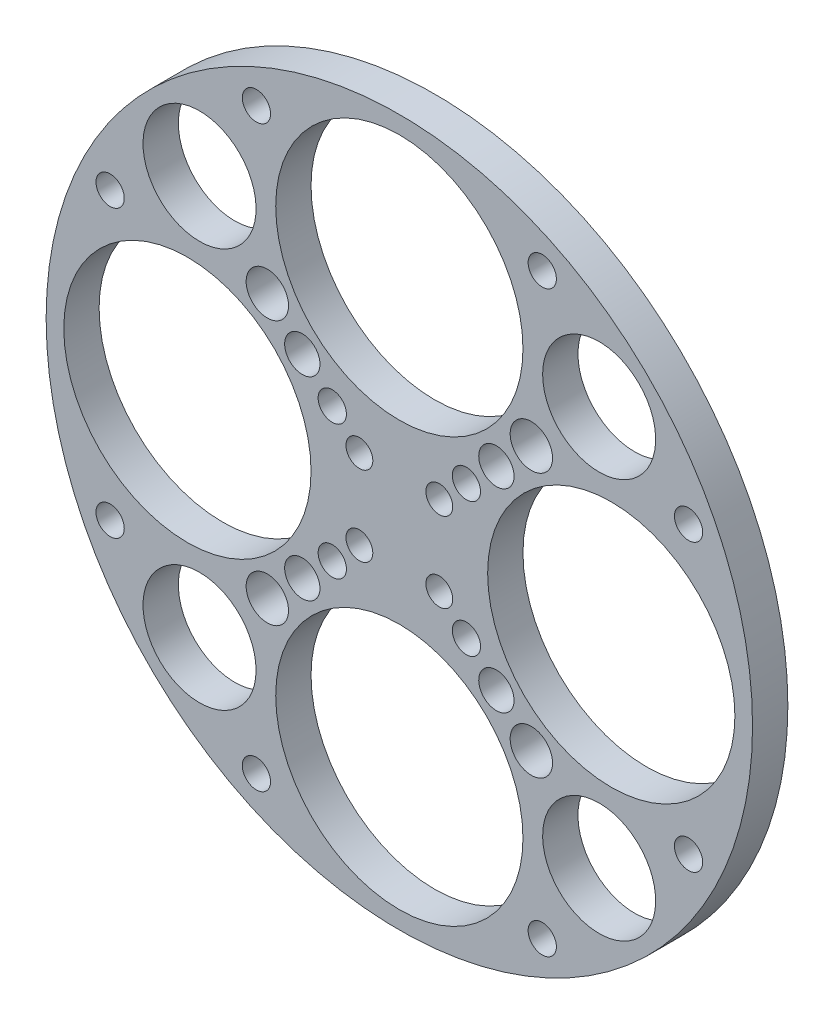
SolidWorks part; units mm, degrees
material "Acrylic (Medium-high impact)"
ref_plane "Front Plane" through (0, 0, 0) normal (0, 0, 1) x (1, 0, 0)
ref_plane "Top Plane" through (0, 0, 0) normal (0, 1, 0) x (1, 0, 0)
ref_plane "Right Plane" through (0, 0, 0) normal (1, 0, 0) x (0, 0, -1)
sketch "Sketch1" plane through (0, 0, 0) normal (0, 0, 1) x (1, 0, 0)
  circle A0 centre (0, 0) radius 50
  dimension "D1" = 100
extrude "Boss-Extrude1" add sketch "Sketch1" along normal blind 5
sketch "Sketch2" plane through (0, 0, 0) normal (0, 0, -1) x (-1, 0, 0)
  line L0 (0, 0) -> (0, 50) construction
  line L1 (-5.6569, 5.6569) -> (0, 0) construction
  circle A0 centre (-5.6569, 5.6569) radius 1.9
  circle A1 centre (0, 0) radius 50 construction
  dimension "D1" = 3.8
  dimension "D2" = 8
  dimension "D3" = 45
extrude "Cut-Extrude1" cut sketch "Sketch2" against normal through all
pattern_circular "CirPattern1" count 4 over 360 about axis through (0, 0, 0) along (0, 0, 1) of "Cut-Extrude1"
sketch "Sketch3" plane through (0, 0, 0) normal (0, 0, -1) x (-1, 0, 0)
  circle A0 centre (0, 30) radius 17.5
  circle A1 centre (-5.6569, 5.6569) radius 4 construction
  dimension "D1" = 8
  dimension "D2" = 35
  dimension "D3" = 30
extrude "Cut-Extrude2" cut sketch "Sketch3" against normal through all
pattern_circular "CirPattern2" count 4 over 360 about axis through (0, 0, 0) along (0, 0, 1) of "Cut-Extrude2"
sketch "Sketch4" plane through (0, 0, 0) normal (0, 0, -1) x (-1, 0, 0)
  line L0 (-30, 0) -> (-30, 30) construction
  line L1 (0, 30) -> (-30, 30) construction
  line L2 (-30, 30) -> (0, 0) construction
  circle A0 centre (-28.2843, 28.2843) radius 8
  circle A1 centre (-18.6863, 18.6863) radius 3
  circle A2 centre (-13.7365, 13.7365) radius 2.5
  circle A3 centre (-9.4939, 9.4939) radius 2
  circle A4 centre (-20.2318, 40.9396) radius 2
  circle A5 centre (0, 30) radius 17.5 construction
  circle A6 centre (-40.9396, 20.2318) radius 2
  dimension "D1" = 16
  dimension "D2" = 40
  dimension "D3" = 6
  dimension "D5" = 5
  dimension "D6" = 7
  dimension "D7" = 4
  dimension "D8" = 6
  dimension "D9" = 4
  dimension "D10" = 23
  dimension "D11" = 15
  dimension "D12" = 4
  dimension "D13" = 15
  dimension "D14" = 23
  dimension "D4" = 16
extrude "Cut-Extrude3" cut sketch "Sketch4" against normal through all
pattern_circular "CirPattern3" count 4 over 360 about axis through (0, 0, 0) along (0, 0, 1) of "Cut-Extrude3"
